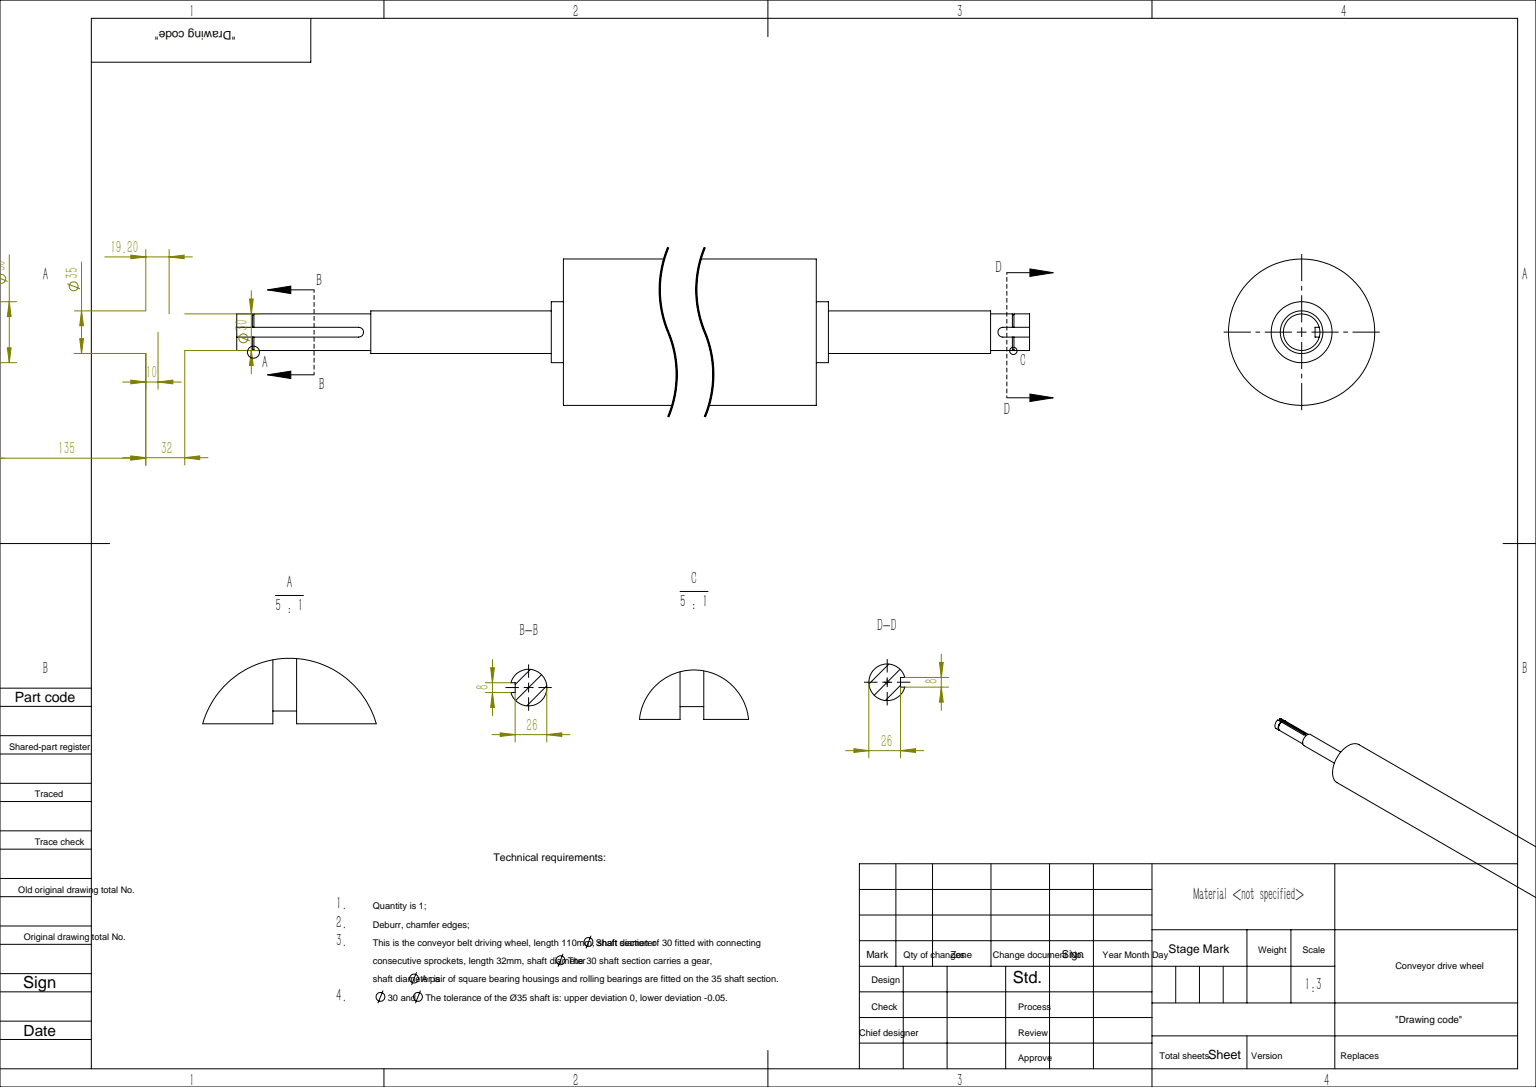
SolidWorks part; units mm, degrees
ref_plane "前视基准面" through (0, 0, 0) normal (0, 0, 1) x (1, 0, 0)
ref_plane "上视基准面" through (0, 0, 0) normal (0, 1, 0) x (1, 0, 0)
ref_plane "右视基准面" through (0, 0, 0) normal (1, 0, 0) x (0, 0, -1)
sketch "草图1" plane through (0, 0, 0) normal (0, 0, 1) x (1, 0, 0)
  line L0 (0, 0) -> (0, 15)
  line L1 (0, 15) -> (110, 15)
  line L2 (110, 15) -> (110, 17.5)
  line L3 (110, 17.5) -> (258, 17.5)
  line L4 (258, 17.5) -> (258, 25)
  line L5 (258, 25) -> (268, 25)
  line L6 (0, 0) -> (1293, 0)
  line L7 (268, 25) -> (268, 60)
  line L8 (268, 60) -> (1118, 60)
  line L9 (1118, 60) -> (1118, 25)
  line L10 (1118, 25) -> (1128, 25)
  line L11 (1128, 25) -> (1128, 17.5)
  line L12 (1128, 17.5) -> (1261, 17.5)
  line L13 (1261, 17.5) -> (1261, 15)
  line L14 (1261, 15) -> (1293, 15)
  line L15 (1293, 15) -> (1293, 0)
  dimension "D1" = 110
  dimension "D2" = 15
  dimension "D3" = 17.5
  dimension "D4" = 148
  dimension "D5" = 10
  dimension "D6" = 25
  dimension "D7" = 60
  dimension "D8" = 850
  dimension "D9" = 10
  dimension "D10" = 25
  dimension "D11" = 17.5
  dimension "D12" = 133
  dimension "D13" = 32
  dimension "D14" = 15
revolve "旋转1" add sketch "草图1" angle 360 about L6
ref_plane "基准面1" through (0, 15, 0) normal (0, 1, 0) x (1, 0, 0)
sketch "草图2" plane through (0, 15, 0) normal (0, 1, 0) x (1, 0, 0)
  line L0 (0, 0) -> (110, 0) construction
  line L1 (110, 17.5) -> (110, -17.5) construction
  line L2 (100, 4) -> (-10, 4)
  line L3 (-10, 4) -> (-10, -4)
  line L4 (-10, -4) -> (100, -4)
  line L5 (110, 15) -> (110, -15) construction
  line L6 (0, 15) -> (0, -15) construction
  arc A0 (100, -4) -> (100, 4) centre (100, 0) ccw
  dimension "D1" = 4
  dimension "D2" = 10
  dimension "D3" = 10
extrude "切除-拉伸1" cut sketch "草图2" against normal blind 4
ref_plane "基准面2" through (12.8, 0, 0) normal (-1, 0, 0) x (0, 0, 1)
sketch "草图3" plane through (12.8, 0, 0) normal (-1, 0, 0) x (0, 0, 1)
  circle A0 centre (0, 0) radius 15
  arc A2 (-4, 14.4568) -> (4, 14.4568) centre (0, 0) ccw construction
  circle A3 centre (0, 0) radius 14.3
  dimension "D1" = 28.6
extrude "切除-拉伸2" cut sketch "草图3" against normal blind 1.3
ref_plane "基准面3" through (0, 15, 0) normal (0, 1, 0) x (1, 0, 0)
sketch "草图4" plane through (0, 15, 0) normal (0, 1, 0) x (1, 0, 0)
  line L0 (1261, 0) -> (1293, 0) construction
  line L1 (1261, -15) -> (1261, 15) construction
  line L2 (1293, -15) -> (1293, 15) construction
  line L3 (1271, 4) -> (1303, 4)
  line L4 (1303, 4) -> (1303, -4)
  line L5 (1303, -4) -> (1271, -4)
  line L6 (1261, -17.5) -> (1261, 17.5) construction
  arc A0 (1271, 4) -> (1271, -4) centre (1271, 0) ccw
  dimension "D1" = 10
  dimension "D2" = 4
  dimension "D3" = 10
extrude "切除-拉伸3" cut sketch "草图4" against normal blind 4
ref_plane "基准面4" through (1280.2, 0, 0) normal (1, 0, 0) x (0, 0, -1)
sketch "草图5" plane through (1280.2, 0, 0) normal (1, 0, 0) x (0, 0, -1)
  circle A0 centre (0, 0) radius 15
  arc A1 (-4, 14.4568) -> (4, 14.4568) centre (0, 0) ccw construction
  circle A2 centre (0, 0) radius 14.3
  dimension "D1" = 28.6
extrude "切除-拉伸4" cut sketch "草图5" against normal blind 1.3
